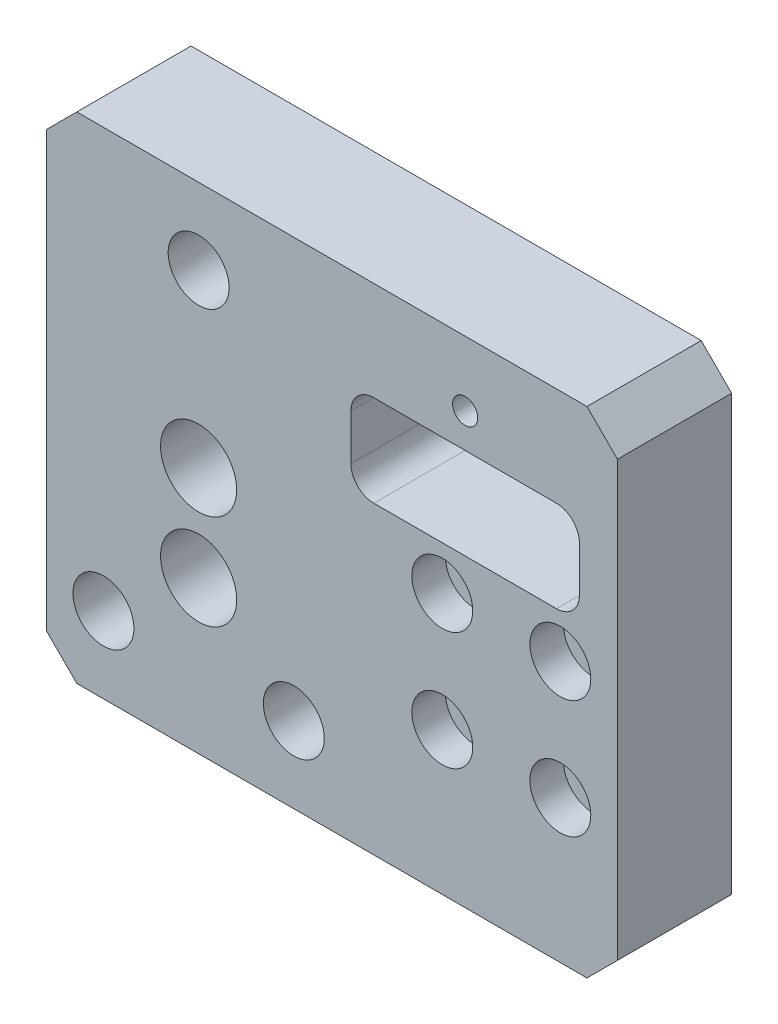
from build123d import *

# Parameters (mm, degrees)
SKETCH_1_W                   = 75
SKETCH_1_H                   = 65
EXTRUDE_1_DEPTH              = 7.5
HOLE_WIZARD_M4_1_D           = 4.5
HOLE_WIZARD_M4_1_CBORE_D     = 8
HOLE_WIZARD_M4_1_CBORE_DEPTH = 4.4
HOLE_WIZARD_8_0_8_1_D        = 8
HOLE_WIZARD_1_D              = 4.5
HOLE_WIZARD_1_CBORE_D        = 10
HOLE_WIZARD_1_CBORE_DEPTH    = 7.5
SKETCH_8_R                   = 4
CUT_EXTRUDE_1_DEPTH          = 4.5
CHAMFER_1_SIZE               = 4
SKETCH_9_W                   = 30
SKETCH_9_H                   = 12
CUT_EXTRUDE_2_DEPTH          = 52.841103383
HOLE_WIZARD_M4_1_2_D         = 3.3
FILLET_1_R                   = 3


with BuildPart() as part:
    # 草图1 → 凸台-拉伸1 (new, symmetric)
    with BuildSketch(Plane.XY):
        Rectangle(SKETCH_1_W, SKETCH_1_H)
    extrude(amount=EXTRUDE_1_DEPTH, both=True)

    # Hole Wizard M4 _1 (through all)
    with Locations(Plane.XY.offset(7.5)):
        with Locations((14.5, 1.75), (14.5, -13.75), (30, 1.75), (30, -13.75)):
            CounterBoreHole(HOLE_WIZARD_M4_1_D / 2, HOLE_WIZARD_M4_1_CBORE_D / 2, HOLE_WIZARD_M4_1_CBORE_DEPTH)

    # Ø8.0 (8) 直径孔1 (through all)
    with Locations(Plane.XY.offset(7.5)):
        with Locations((-17.5, 22.5), (-30, -22.5), (-5, -22.5)):
            Hole(HOLE_WIZARD_8_0_8_1_D / 2)

    # 孔1 (through all)
    with Locations(Plane.XY.offset(7.5)):
        with Locations((-17.5, 0), (-17.5, -12.5)):
            CounterBoreHole(HOLE_WIZARD_1_D / 2, HOLE_WIZARD_1_CBORE_D / 2, HOLE_WIZARD_1_CBORE_DEPTH)

    # 草图8 → 切除-拉伸1 (cut)
    with BuildSketch(Plane(origin=(0, 0, -7.5), x_dir=(-1, 0, 0), z_dir=(0, 0, -1))):
        with Locations((17.5, 0)):
            Circle(SKETCH_8_R)
        with Locations((17.5, -12.5)):
            Circle(SKETCH_8_R)
    extrude(amount=-CUT_EXTRUDE_1_DEPTH, mode=Mode.SUBTRACT)

    # 倒角1
    chamfer_1_edges = [part.edges().sort_by_distance(p)[0] for p in [
        (37.5, -32.5, 0),
        (-37.5, -32.5, 0),
        (-37.5, 32.5, 0),
        (37.5, 32.5, 0),
    ]]
    chamfer(chamfer_1_edges, length=CHAMFER_1_SIZE)

    # 草图9 → 切除-拉伸2 (cut, through all)
    with BuildSketch(Plane(origin=(0, 0, -7.5), x_dir=(-1, 0, 0), z_dir=(0, 0, -1))):
        with Locations((-17.5, 13.5)):
            Rectangle(SKETCH_9_W, SKETCH_9_H)
    extrude(amount=-CUT_EXTRUDE_2_DEPTH, mode=Mode.SUBTRACT)

    # Hole Wizard M4 _1 2 (through all)
    with Locations(Plane(origin=(0, 0, -7.5), x_dir=(-1, 0, 0), z_dir=(0, 0, -1))):
        with Locations((-17.5, 24)):
            Hole(HOLE_WIZARD_M4_1_2_D / 2)

    # 圆角1
    fillet_1_edges = [part.edges().sort_by_distance(p)[0] for p in [
        (2.5, 19.5, 0),
        (2.5, 7.5, 0),
        (32.5, 7.5, 0),
        (32.5, 19.5, 0),
    ]]
    fillet(fillet_1_edges, radius=FILLET_1_R)


solid = part.part
